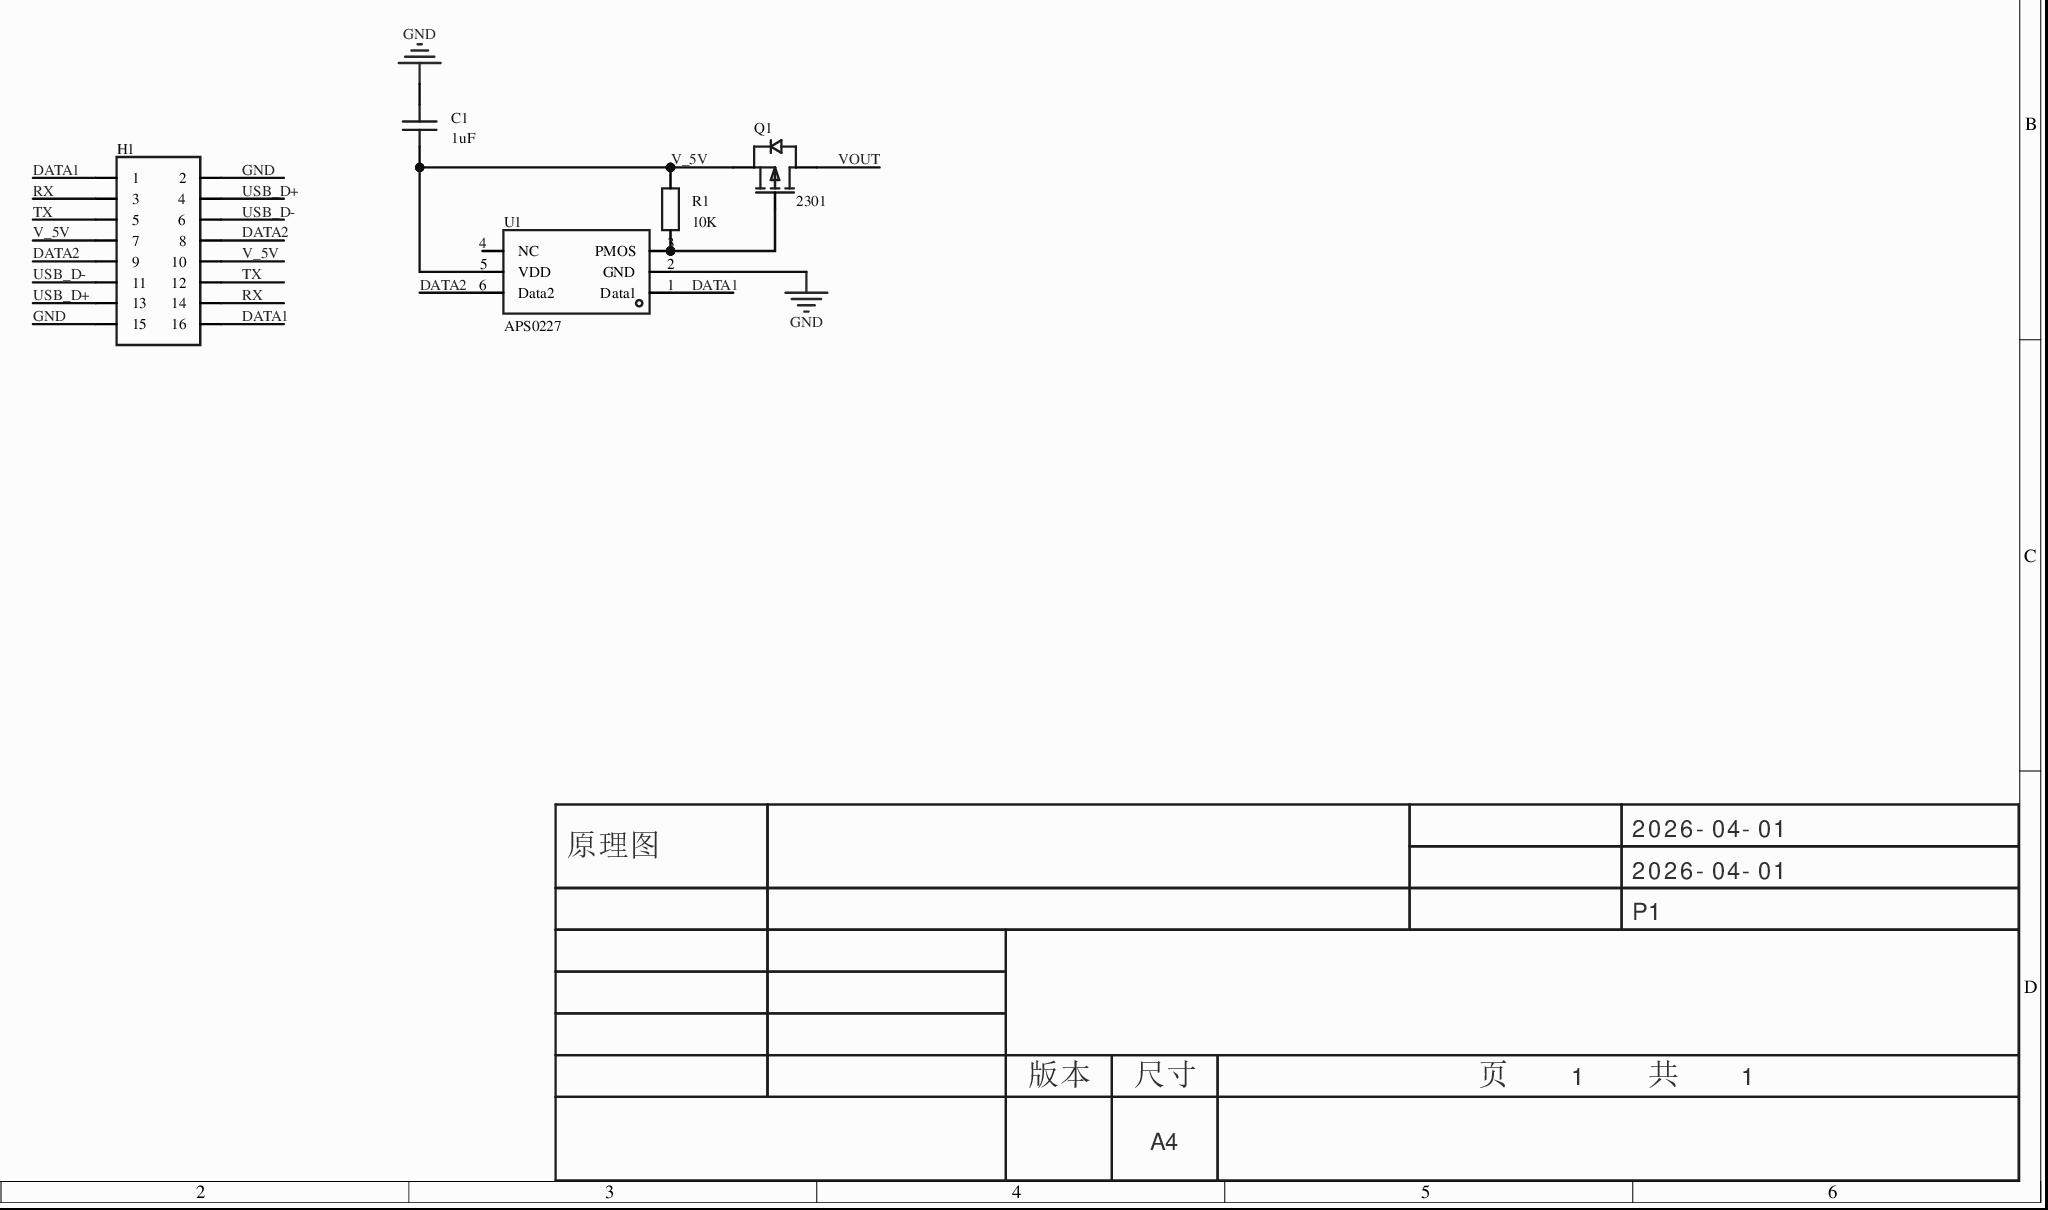
[diagram p0: MISC52013-3.schdoc]
# Altium project MISC52013-2.PrjPcb
1 sheet, 5 parts. Net scope: global (net labels, ports and power ports of the same name join across sheets).
Board file: MISC52013.pcbdoc

## Sheet MISC52013-3.schdoc
size 297 x 209 mm; Version: V1.0; @Project Name: MISC52013; @Update Date: 2026-04-01; @Create Date: 2026-04-01; @Board Name: MISC52013; @Create Time: 13:53:31; @Page Count: 1; @Page No: 1; @Schematic Name: MISC52013; @Update Time: 13:53:31; Size: A4

### Parts
C1  1uF  [C0402]
H1  (no value)  [HDR-TH_16P-P2.54-V-F-R2-C8-S2.54-1]
Q1  2301  [SOT-23-3_L3.0-W1.7-P0.95-LS2.9-BR]
R1  10K  [R0402]
U1  APS0227  [TSOT-23-6_L2.9-W1.6-P0.95-LS2.8-BR]

### Nets
GND: C1.2 H1.2 H1.15 U1.2(GND)
DATA1: H1.1 H1.16 U1.1(Data1)
DATA2: H1.8 H1.9 U1.6(Data2)
RX: H1.3 H1.14
TX: H1.5 H1.12
USB_D+: H1.4 H1.13
USB_D-: H1.6 H1.11
V_5V: C1.1 H1.7 H1.10 Q1.2(S) R1.2 U1.5(VDD)
VOUT: Q1.3(D)
NetQ1_1: Q1.1(G) R1.1 U1.3(PMOS)

Not connected (* = marked no-connect by the designer): U1 4(NC)*

### Notes on the sheet
- 2026-04-01
- 原理图
- P1
- 版本
- 尺寸
- A4
- 页    1    共    1

### Library data of the parts
C1 = CAP_0402: Symbol: Capacitance; ConvertToPcb: yes; ModelId: 36a51122f27c49738f86b3bfa98863e00819f05c4eef4c71ace90d822a990e87; ModelName: C0402_L1.0-W0.5-H0.5; ModelTransform: 39.37,19.685,0,0,0,0,0,0,0; Device: CAP_0402; Value: 1uF; AddInBom: yes; Supplier Footprint: 0402; FootprintName: C0402
H1 = HDR-F_2.54_2x8: Symbol: HDR-F-2.54_2x8; ConvertToPcb: yes; ModelId: f6b5f7d40ec74b809fbaeebc5002f6e00819f05c4eef4c71ace90d822a990e87; ModelName: HDR2.54-F-LI-2X8P; ModelTransform: 799.99844,200,0,0,0,0,0,0,-118.11; Device: HDR-F_2.54_2x8; AddInBom: yes; SupplierPart: C30734; Supplier Footprint: 插件; FootprintName: HDR-TH_16P-P2.54-V-F-R2-C8-S2.54-1
Q1 = SI2301CDS-T1-GE3: 数量:1个P沟道;漏源电压(Vdss):20V;连续漏极电流(Id):3.1A;导通电阻(RDS(on)):142mΩ@2.5V,2.7A;耗散功率(Pd):1.6W;阈值电压(Vgs(th)):1V@250uA;; Manufacturer: VISHAY(威世); AddInBom: yes; ModelId: 89cb27a44ab2466697082bb9fd73a7d00819f05c4eef4c71ace90d822a990e87; ModelName: SOT-23-3L_L2.9-W1.6-H1.1-LS2.8-P0.95; ModelTransform: 114.173,110.236,0,90,0,0,0,0,0; Number: 1个P沟道; Drain to Source Voltage: 20V; Current - Continuous Drain(Id): 3.1A; Pd - Power Dissipation: 1.6W; Gate Charge(Qg): 10nC@4.5V; Input Capacitance(Ciss): 405pF; Reverse Transfer Capacitance (Crss@Vds): 55pF; Type: P沟道; Output Capacitance(Coss): 75pF; Symbol: SI2301CDS-T1-GE3; Device: SI2301CDS-T1-GE3; Manufacturer Part: 2301; LCSC Part Name: 1个P沟道 耐压:20V 电流:3.1A; SupplierPart: C10487; Supplier Footprint: SOT-23; JLCPCB Part Class: Basic Part; Datasheet: https://item.szlcsc.com/datasheet/SI2301CDS-T1-GE3/11030.html; Supplier: LCSC; ConvertToPcb: yes; FootprintName: SOT-23-3_L3.0-W1.7-P0.95-LS2.9-BR; RDS(on): 142mΩ@2.5V,2.7A; Gate Threshold Voltage (Vgs(th)): 1V@250uA; Operating Temperature: -55℃~+150℃
R1 = Res_0402: Symbol: 电阻; ConvertToPcb: yes; ModelId: 98c88bc2b9094f218f3a3e30a70127380819f05c4eef4c71ace90d822a990e87; ModelName: R0402_L1.0-W0.5-H0.4; ModelTransform: 39.37,19.685,0,0,0,0,0,0,0; Device: Res_0402; AddInBom: yes; Supplier Footprint: 0402; FootprintName: R0402; Value: 10K
U1 = APS0227: AddInBom: yes; ModelId: 2c4039b5b88644c1bda4b4ba9e9716670819f05c4eef4c71ace90d822a990e87; ModelName: TSOT-23-6_L2.9-W1.6-H1.1-LS2.8-P0.95; ModelTransform: 110.45568,114.173,0,180,0,0,-0.005,-0.0005,0; Symbol: APS0227; Device: APS0227; LCSC Part Name: APS0227; SupplierPart: C9900264825; ManufacturerPart: APS0227; Supplier Footprint: sot-23-6L; Supplier: LCSC; ConvertToPcb: yes; FootprintName: TSOT-23-6_L2.9-W1.6-P0.95-LS2.8-BR